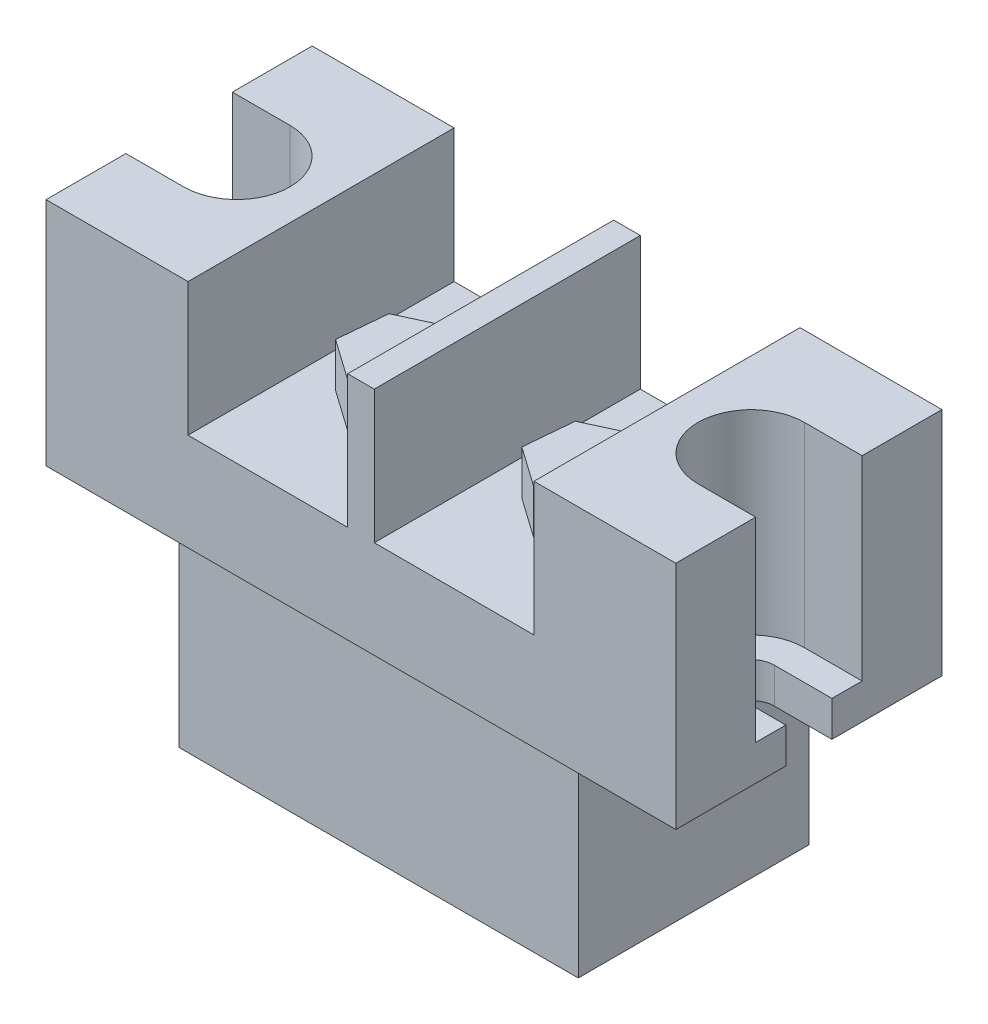
SolidWorks part; units mm, degrees
ref_plane "前视基准面" through (0, 0, 0) normal (0, 0, 1) x (1, 0, 0)
ref_plane "上视基准面" through (0, 0, 0) normal (0, 1, 0) x (1, 0, 0)
ref_plane "右视基准面" through (0, 0, 0) normal (1, 0, 0) x (0, 0, -1)
sketch "草图1" plane through (0, 0, 0) normal (0, 1, 0) x (1, 0, 0)
  line L1 (-35.5, 15) -> (35.5, 15)
  line L2 (-35.5, 15) -> (-35.5, -15)
  line L3 (-35.5, -15) -> (35.5, -15)
  line L4 (35.5, 15) -> (35.5, -15)
  line L5 (-35.5, 15) -> (35.5, -15) construction
  line L6 (-35.5, -15) -> (35.5, 15) construction
  point P0 (0, 0)
  dimension "D1" = 71
  dimension "D2" = 30
extrude "凸台-拉伸1" add sketch "草图1" along normal blind 26
sketch "草图2" plane through (0, 0, 0) normal (0, -1, 0) x (1, 0, 0)
  line L1 (-22.5, 13) -> (22.5, 13)
  line L2 (-22.5, 13) -> (-22.5, -13)
  line L3 (-22.5, -13) -> (22.5, -13)
  line L4 (22.5, 13) -> (22.5, -13)
  line L5 (-22.5, 13) -> (22.5, -13) construction
  line L6 (-22.5, -13) -> (22.5, 13) construction
  point P0 (0, 0)
  dimension "D1" = 45
  dimension "D2" = 26
extrude "凸台-拉伸2" add sketch "草图2" along normal blind 22
sketch "草图3" plane through (0, 26, 0) normal (0, 1, 0) x (1, 0, 0)
  line L0 (-29, 0) -> (29, 0) construction
  line L1 (-29, 0) -> (-61.7002, 0) construction
  line L3 (-29, -2.6) -> (-61.7002, -2.6)
  line L4 (-29, 2.6) -> (-61.7002, 2.6)
  line L5 (29, 0) -> (61.7002, 0) construction
  line L6 (29, 2.6) -> (61.7002, 2.6)
  line L7 (29, -2.6) -> (61.7002, -2.6)
  arc A0 (-29, -2.6) -> (-29, 2.6) centre (-29, 0) ccw
  arc A1 (-61.7002, 2.6) -> (-61.7002, -2.6) centre (-61.7002, 0) ccw
  arc A2 (29, 2.6) -> (29, -2.6) centre (29, 0) ccw
  arc A3 (61.7002, -2.6) -> (61.7002, 2.6) centre (61.7002, 0) ccw
  point P2 (-45.3501, 0)
  point P11 (45.3501, 0)
  dimension "D1" = 58
  dimension "D2" = 5.2
extrude "切除-拉伸1" cut sketch "草图3" against normal through all
sketch "草图4" plane through (0, 26, 0) normal (0, 1, 0) x (1, 0, 0)
  line L0 (29, 0) -> (52.5138, 0) construction
  line L1 (29, 6) -> (52.5138, 6)
  line L2 (29, -6) -> (52.5138, -6)
  line L3 (-29, 0) -> (-53.0072, 0) construction
  line L4 (-29, -6) -> (-53.0072, -6)
  line L5 (-29, 6) -> (-53.0072, 6)
  arc A0 (29, 6) -> (29, -6) centre (29, 0) ccw
  arc A1 (52.5138, -6) -> (52.5138, 6) centre (52.5138, 0) ccw
  arc A2 (-29, -6) -> (-29, 6) centre (-29, 0) ccw
  arc A3 (-53.0072, 6) -> (-53.0072, -6) centre (-53.0072, 0) ccw
  point P4 (40.7569, 0)
  point P9 (-41.0036, 0)
  dimension "D1" = 6
  dimension "D2" = 6
extrude "切除-拉伸2" cut sketch "草图4" against normal offset from surface (22 mm away) 4 up to face at (0, 0, 0)
sketch "草图5" plane through (0, 26, 0) normal (0, 1, 0) x (1, 0, 0)
  line L1 (1.5, 15) -> (19.5, 15)
  line L2 (1.5, 15) -> (1.5, -15)
  line L3 (1.5, -15) -> (19.5, -15)
  line L4 (19.5, 15) -> (19.5, -15)
  line L5 (-35.5, -15) -> (35.5, -15) construction
  line L6 (10.5, 15) -> (10.5, -0.6921) construction
  line L8 (35.5, 15) -> (-35.5, 15) construction
  dimension "D1" = 18
  dimension "D2" = 15.6921
  dimension "D3" = 10.5
extrude "切除-拉伸3" cut sketch "草图5" against normal blind 15
pattern_linear "阵列(线性)1" count 2 spacing 21 along (-1, 0, 0) of "切除-拉伸3"
sketch "草图6" plane through (0, 11, 0) normal (0, 1, 0) x (1, 0, 0)
  line L0 (10.5, 15) -> (10.5, 0) construction
  line L2 (10.5, 0) -> (0, 0) construction
  line L3 (19.5, 15) -> (1.5, 15) construction
  line L4 (15.033, -3.1957) -> (15.5341, 2.3279)
  line L5 (15.5341, 2.3279) -> (11.0011, 5.5236)
  line L6 (11.0011, 5.5236) -> (5.967, 3.1957)
  line L7 (5.967, 3.1957) -> (5.4659, -2.3279)
  line L8 (5.4659, -2.3279) -> (9.9989, -5.5236)
  line L9 (9.9989, -5.5236) -> (15.033, -3.1957)
  circle A0 centre (10.5, 0) radius 4.8032 construction
  dimension "D1" = 9.6064
extrude "凸台-拉伸3" add sketch "草图6" along normal blind 5
pattern_linear "阵列(线性)2" count 2 spacing 21 along (-1, 0, 0) of "凸台-拉伸3"
